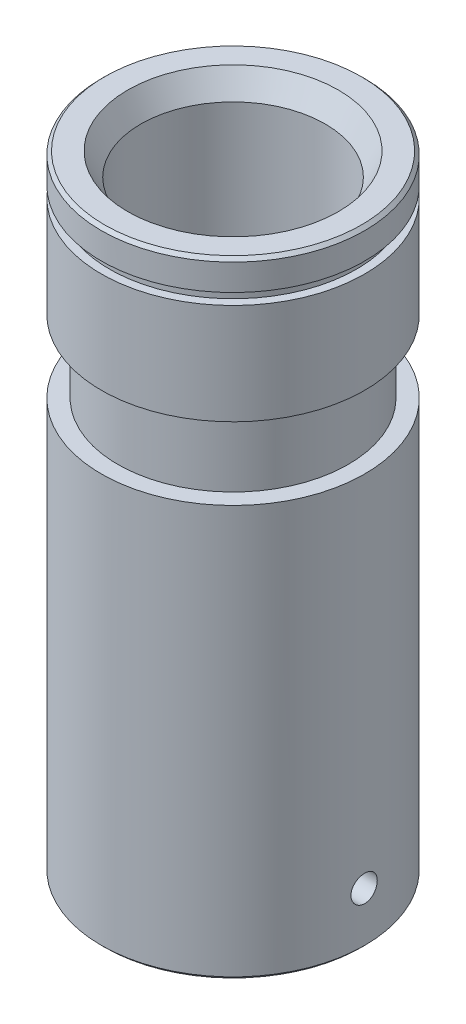
SolidWorks part; units mm, degrees
ref_plane "前视基准面" through (0, 0, 0) normal (0, 0, 1) x (1, 0, 0)
ref_plane "上视基准面" through (0, 0, 0) normal (0, 1, 0) x (1, 0, 0)
ref_plane "右视基准面" through (0, 0, 0) normal (1, 0, 0) x (0, 0, -1)
sketch "草图1" plane through (0, 0, 0) normal (0, 1, 0) x (1, 0, 0)
  circle A0 centre (0, 0) radius 20
  circle A1 centre (0, 0) radius 14
  dimension "D1" = 40
  dimension "D2" = 28
extrude "凸台-拉伸1" add sketch "草图1" along normal blind 95
sketch "草图3" plane through (0, 0, 0) normal (0, 0, 1) x (1, 0, 0)
  line L0 (20, 0) -> (20, 95) construction
  line L1 (20, 73.5) -> (17.5, 73.5)
  line L2 (20, 73.5) -> (20, 62.5)
  line L3 (20, 62.5) -> (17.5, 62.5)
  line L4 (17.5, 73.5) -> (17.5, 62.5)
  line L5 (0, 0) -> (0, 18.6447) construction
  line L6 (20, 95) -> (-20, 95) construction
  line L8 (20, 90.5) -> (18.75, 90.5)
  line L9 (20, 90.5) -> (20, 88.8)
  line L10 (20, 88.8) -> (18.75, 88.8)
  line L11 (18.75, 90.5) -> (18.75, 88.8)
  dimension "D1" = 11
  dimension "D2" = 17.5
  dimension "D3" = 21.5
  dimension "D4" = 1.7
  dimension "D5" = 18.75
  dimension "D6" = 4.5
revolve "切除-旋转1" cut sketch "草图3" angle 360 about L5
sketch "草图4" plane through (0, 0, 0) normal (0, -1, 0) x (1, 0, 0)
  circle A0 centre (0, 0) radius 14 construction
  circle A1 centre (0, 0) radius 14
  circle A2 centre (0, 0) radius 11
  dimension "D1" = 22
extrude "凸台-拉伸2" add sketch "草图4" against normal blind 14
chamfer "倒角1" distance 0.5 angle 45 2 edges at (0, 95, 20) (0, 0, 20)
hole_wizard "Ø4.0 (4) 直径孔3" positions "3D草图2" profile "草图6" hole size "Ø4.0" standard "GB" end condition through all
sketch3d "3D草图2"
  point P0 (20, 8, 0)
  dimension "D1" = 8
sketch "草图6" plane through (20, 8, 0) normal (0, 1, 0) x (0, 0, -1)
  line L0 (0, 0) -> (0, 40)
  line L1 (0, 40) -> (2, 40)
  line L2 (2, 40) -> (2, 0)
  line L5 (2, 0) -> (0, 0)
  line L11 (0, -6.35) -> (0, 107.95) construction
  dimension "通孔孔直径" = 4
  dimension "通孔孔深度" = 40
sketch "草图7" plane through (0, 0, 0) normal (0, 0, 1) x (1, 0, 0)
  line L0 (-19.5, 0) -> (19.5, 0) construction
  line L1 (-20, 40) -> (-18, 40)
  line L2 (-20, 40) -> (-20, 30)
  line L3 (-20, 30) -> (-18, 30)
  line L4 (-18, 40) -> (-18, 30)
  line L5 (-20, 62.5) -> (-20, 10) construction
  dimension "D1" = 2
  dimension "D2" = 10
  dimension "D3" = 30
extrude "切除-拉伸1" cut sketch "草图7" against normal mid plane 20
chamfer "倒角2" distance 2 angle 60 2 edges at (0, 0, -11) (0, 95, 14)
